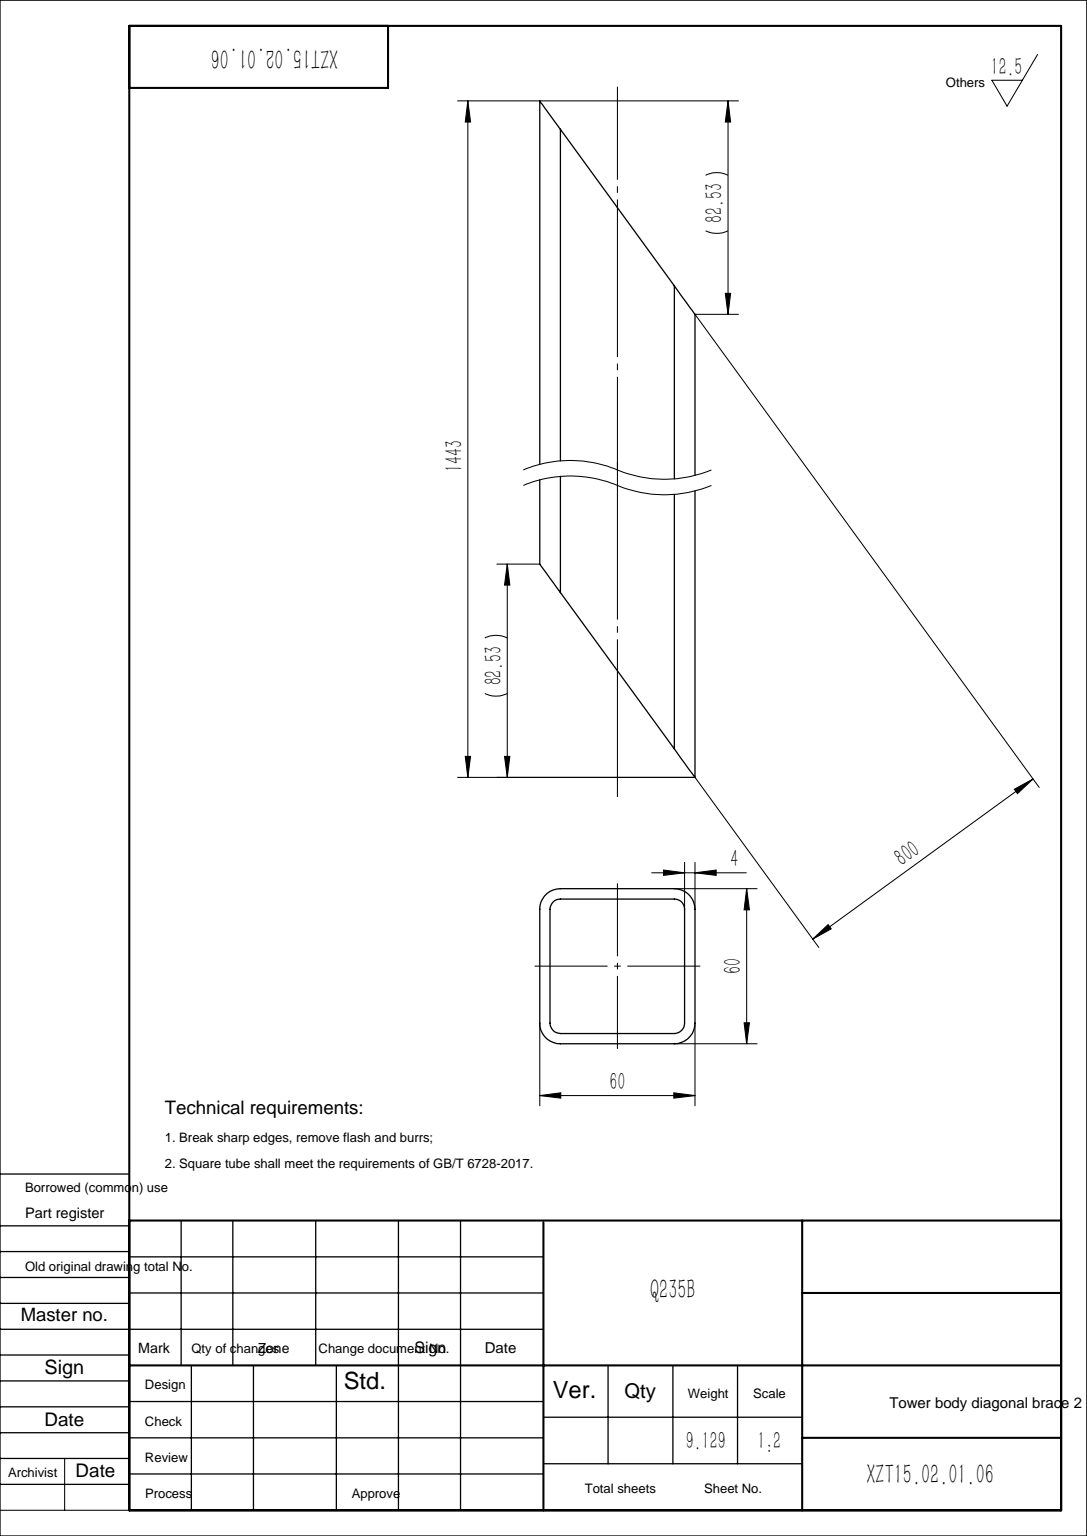
from build123d import *

# Parameters (mm, degrees)
GB_T_6728_2002_SQUARE_HOLLOW_SECTION_60_DEPTH = 1443
CUT_EXTRUDE1_DEPTH                            = 1445.558410034
CUT_EXTRUDE1_DEPTH_BACK                       = 1445.558410034


with BuildPart() as part:
    # Sketch1 → GB/T 6728-2002 square hollow section 60×60×4(1) (new body)
    with BuildSketch(Plane(origin=(0, 0, 0), x_dir=(-1, 0, 0), z_dir=(0, 1, 0))):
        with BuildLine():
            Line((-22, -30), (22, -30))
            ThreePointArc((22, -30), (27.656854249, -27.656854249), (30, -22))
            Line((30, -22), (30, 22))
            ThreePointArc((30, 22), (27.656854249, 27.656854249), (22, 30))
            Line((22, 30), (-22, 30))
            ThreePointArc((-22, 30), (-27.656854249, 27.656854249), (-30, 22))
            Line((-30, 22), (-30, -22))
            ThreePointArc((-30, -22), (-27.656854249, -27.656854249), (-22, -30))
        make_face()
        with BuildLine():
            Line((-22, -26), (22, -26))
            ThreePointArc((22, -26), (24.828427125, -24.828427125), (26, -22))
            Line((26, -22), (26, 22))
            ThreePointArc((26, 22), (24.828427125, 24.828427125), (22, 26))
            Line((22, 26), (-22, 26))
            ThreePointArc((-22, 26), (-24.828427125, 24.828427125), (-26, 22))
            Line((-26, 22), (-26, -22))
            ThreePointArc((-26, -22), (-24.828427125, -24.828427125), (-22, -26))
        make_face(mode=Mode.SUBTRACT)
    extrude(amount=GB_T_6728_2002_SQUARE_HOLLOW_SECTION_60_DEPTH)

    # Sketch2 → Cut-Extrude1 (cut, two sides: drawn at the far end of the back side and taken through both)
    with BuildSketch(Plane.XY.offset(30).offset(-CUT_EXTRUDE1_DEPTH_BACK)):
        Polygon((-30, 1443), (30, 1360.470047999), (30, 1443), align=None)
        Polygon((-30, 0), (-30, 82.529952001), (30, 0), align=None)
    extrude(amount=CUT_EXTRUDE1_DEPTH + CUT_EXTRUDE1_DEPTH_BACK, mode=Mode.SUBTRACT)


solid = part.part
